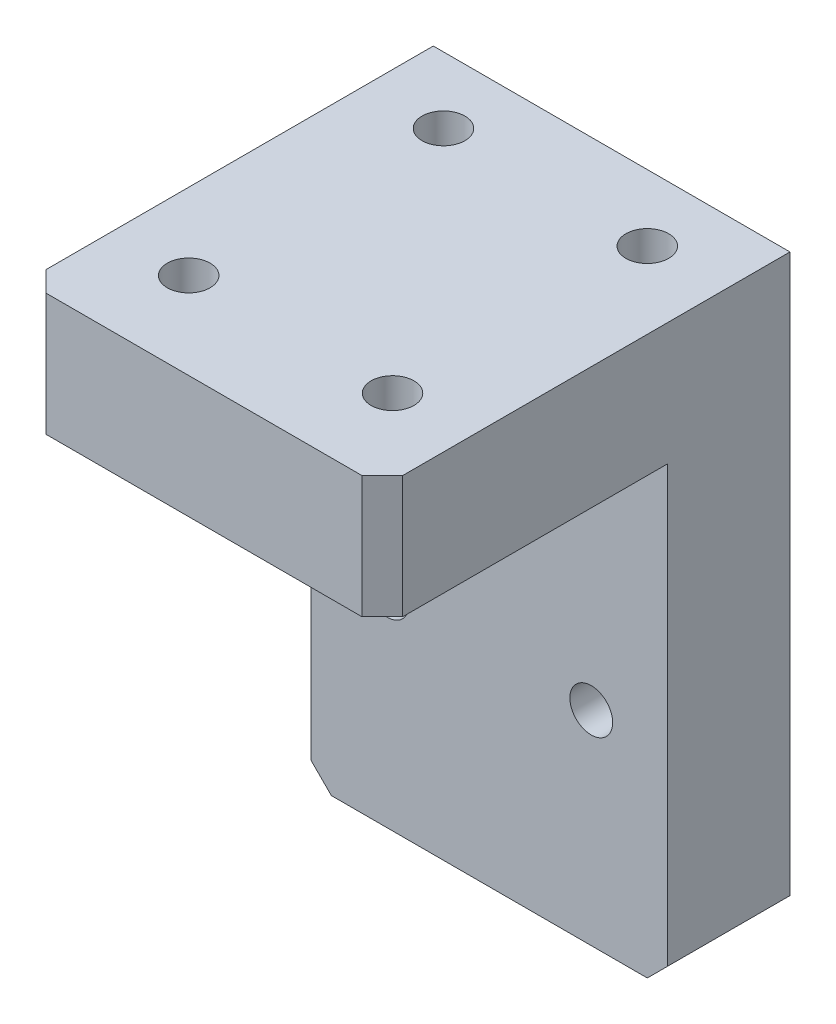
SolidWorks part; units mm, degrees
ref_plane "前视基准面" through (0, 0, 0) normal (0, 0, 1) x (1, 0, 0)
ref_plane "上视基准面" through (0, 0, 0) normal (0, 1, 0) x (1, 0, 0)
ref_plane "右视基准面" through (0, 0, 0) normal (1, 0, 0) x (0, 0, -1)
sketch "草图1" plane through (0, 0, 0) normal (0, 0, 1) x (1, 0, 0)
  line L1 (-17.5, -28.35) -> (17.5, -28.35)
  line L2 (-17.5, -28.35) -> (-17.5, 28.35)
  line L3 (-17.5, 28.35) -> (17.5, 28.35)
  line L4 (17.5, -28.35) -> (17.5, 28.35)
  line L5 (-17.5, -28.35) -> (17.5, 28.35) construction
  line L6 (-17.5, 28.35) -> (17.5, -28.35) construction
  point P0 (0, 0)
  dimension "D1" = 35
  dimension "D2" = 56.7
extrude "凸台-拉伸1" add sketch "草图1" along normal blind 12 contours L3 L4 L1 L2
chamfer "倒角1" distance 2 angle 45 2 edges at (17.5, -28.35, 6) (-17.5, -28.35, 6)
sketch "草图4" plane through (-17.5, 0, 0) normal (-1, 0, 0) x (0, 0, 1)
  line L1 (12, 28.35) -> (40, 28.35)
  line L2 (12, 28.35) -> (12, 16.35)
  line L3 (12, 16.35) -> (40, 16.35)
  line L4 (40, 28.35) -> (40, 16.35)
  line L6 (12, -26.35) -> (12, 28.35) construction
  line L7 (12, 28.35) -> (0, 28.35) construction
  dimension "D1" = 28
  dimension "D2" = 12
extrude "凸台-拉伸2" add sketch "草图4" against normal up to surface (35 mm away) up to face at (17.5, 1, 6)
sketch "草图7" plane through (0, 0, 0) normal (0, 0, -1) x (-1, 0, 0)
  point P11 (-10, -8.35)
  point P14 (10, -8.35)
hole_wizard "M5 螺纹孔1" positions "草图7" profile "草图6" tap size "M5" standard "GB" end condition through all
sketch "草图6" plane through (10, -8.35, 0) normal (1, 0, 0) x (0, 1, 0)
  line L0 (0, 0) -> (0, 40)
  line L1 (0, 40) -> (2.1, 40)
  line L2 (2.1, 40) -> (2.1, 0)
  line L5 (2.1, 0) -> (0, 0)
  line L11 (0, -6.35) -> (0, 107.95) construction
  dimension "通孔螺纹孔钻头直径" = 4.2
  dimension "通孔螺纹孔钻头深度" = 40
cosmetic thread "孔螺纹线1" parameters "D2"=5
cosmetic thread "孔螺纹线8" parameters "D2"=5
chamfer "倒角2" distance 2 angle 45 2 edges at (17.5, 22.35, 40) (-17.5, 22.35, 40)
sketch "草图10" plane through (0, 28.35, 0) normal (0, 1, 0) x (1, 0, 0)
  line L0 (17.5, -19) -> (-35.1832, -19) construction
  line L1 (17.5, -38) -> (17.5, 0) construction
  line L3 (0, -49.559) -> (0, 8.1698) construction
  point P0 (-10, -6.5)
  point P2 (10, -6.5)
  point P4 (-10, -31.5)
  point P6 (10, -31.5)
  dimension "D1" = 25
  dimension "D2" = 20
hole_wizard "M5 螺纹孔2" positions "草图10" profile "草图9" tap size "M5" standard "GB"
sketch "草图9" plane through (-10, 28.35, 6.5) normal (1, 0, 0) x (0, 0, 1)
  line L0 (0, 0) -> (0, 13.6618)
  line L1 (0, 13.6618) -> (2.1, 12.4)
  line L2 (2.1, 12.4) -> (2.1, 0)
  line L5 (2.1, 0) -> (0, 0)
  line L10 (0, 13.6618) -> (-2.1, 12.4) construction
  line L11 (0, -6.35) -> (0, 107.95) construction
  dimension "螺纹孔钻头直径" = 4.2
  dimension "螺纹孔钻头深度" = 12.4
  dimension "导头角度" = 118
cosmetic thread "孔螺纹线3" parameters "D1"=10, "D2"=5
cosmetic thread "孔螺纹线4" parameters "D1"=10, "D2"=5
cosmetic thread "孔螺纹线5" parameters "D1"=10, "D2"=5
cosmetic thread "孔螺纹线6" parameters "D1"=10, "D2"=5
